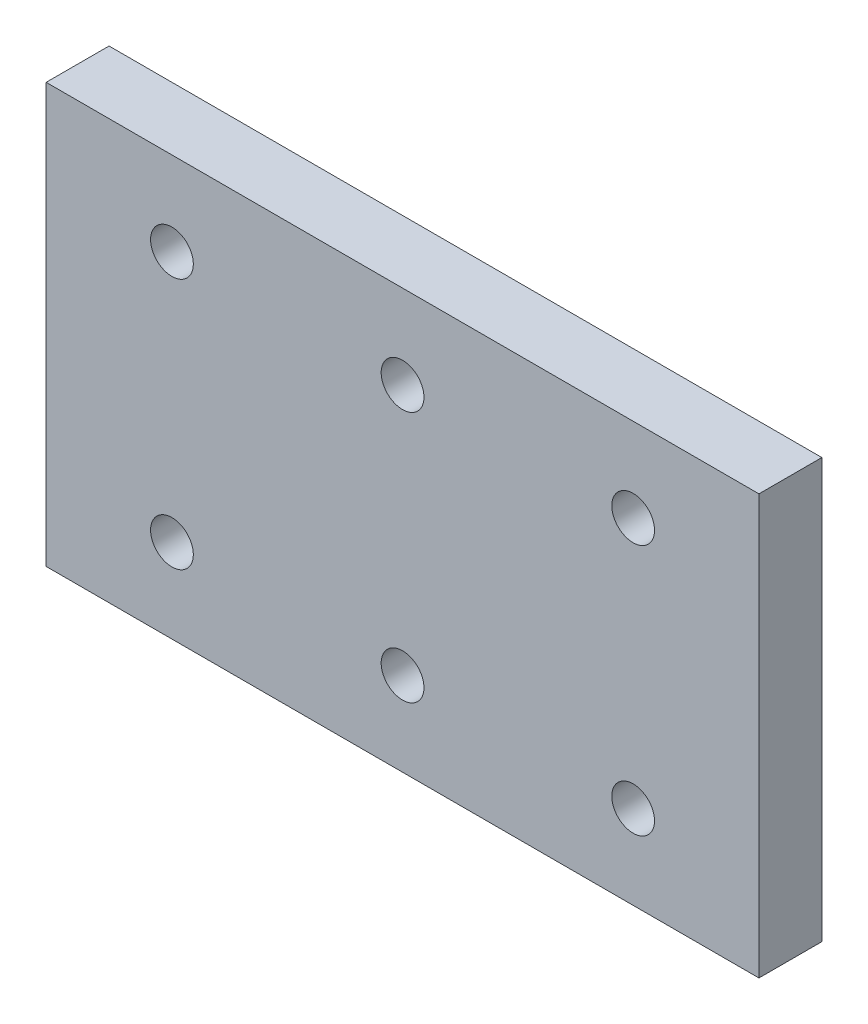
SolidWorks part; units mm, degrees
material "1023 碳钢板 (SS)"
ref_plane "Front Plane" through (0, 0, 0) normal (0, 0, 1) x (1, 0, 0)
ref_plane "Top Plane" through (0, 0, 0) normal (0, 1, 0) x (1, 0, 0)
ref_plane "Right Plane" through (0, 0, 0) normal (1, 0, 0) x (0, 0, -1)
sketch "Sketch1" plane through (0, 0, 0) normal (0, 0, 1) x (1, 0, 0)
  line L1 (85, 50) -> (-85, 50)
  line L2 (85, 50) -> (85, -50)
  line L3 (85, -50) -> (-85, -50)
  line L4 (-85, 50) -> (-85, -50)
  line L5 (85, 50) -> (-85, -50) construction
  line L6 (85, -50) -> (-85, 50) construction
  point P0 (0, 0)
  dimension "D1" = 170
  dimension "D2" = 100
extrude "Boss-Extrude1" add sketch "Sketch1" along normal blind 15 contours L2 L1 L4 L3
sketch "Sketch2" plane through (0, 0, 15) normal (0, 0, 1) x (1, 0, 0)
  line L0 (-85, 50) -> (-85, -50) construction
  circle A0 centre (-55, 30) radius 4.5
  circle A1 centre (-55, -30) radius 4.5
  circle A2 centre (0, 30) radius 4.5
  circle A3 centre (0, -30) radius 4.5
  circle A4 centre (55, 30) radius 4.5
  circle A5 centre (55, -30) radius 4.5
  dimension "D6" = 9
  dimension "D1" = 60
  dimension "D2" = 30
  dimension "D3" = 55
  dimension "D4" = 55
  dimension "D5" = 30
hole_wizard "M12 Tapped Hole1" positions "Sketch3" profile "Sketch4" tap size "M12" standard "ISO"
sketch "Sketch3" plane through (0, 0, 15) normal (0, 0, 1) x (1, 0, 0)
  point P0 (-55, 30)
  point P3 (0, 30)
  point P6 (55, 30)
  point P9 (55, -30)
  point P12 (0, -30)
  point P15 (-55, -30)
sketch "Sketch4" plane through (-55, 30, 15) normal (1, 0, 0) x (0, -1, 0)
  line L0 (0, 0) -> (0, 32.3144)
  line L1 (0, 32.3144) -> (5.1, 29.25)
  line L2 (5.1, 29.25) -> (5.1, 0)
  line L5 (5.1, 0) -> (0, 0)
  line L10 (0, 32.3144) -> (-5.1, 29.25) construction
  line L11 (0, -6.35) -> (0, 107.95) construction
  dimension "螺纹孔钻头直径" = 10.2
  dimension "螺纹孔钻头深度" = 29.25
  dimension "导头角度" = 118
cosmetic thread "Hole Thread Line 1"
cosmetic thread "Hole Thread Line 2"
cosmetic thread "Hole Thread Line 3"
cosmetic thread "Hole Thread Line 4"
cosmetic thread "Hole Thread Line 5"
cosmetic thread "Hole Thread Line 6"
